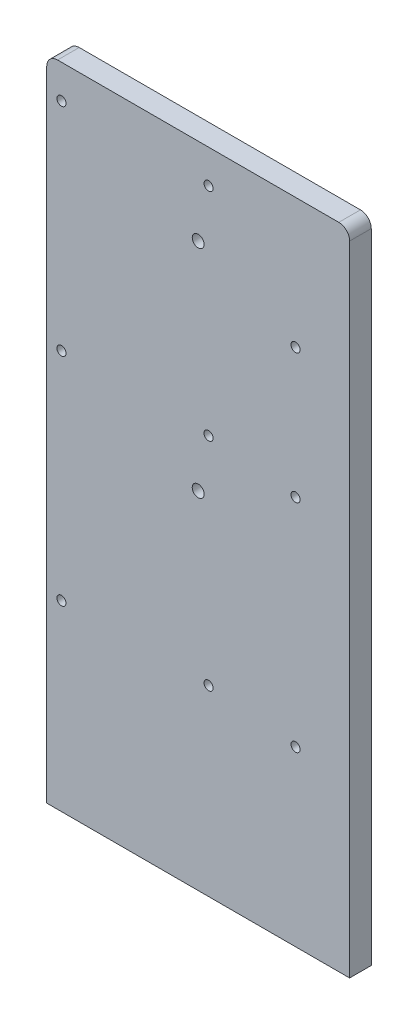
SolidWorks part; units mm, degrees
ref_plane "前视基准面" through (0, 0, 0) normal (0, 0, 1) x (1, 0, 0)
ref_plane "上视基准面" through (0, 0, 0) normal (0, 1, 0) x (1, 0, 0)
ref_plane "右视基准面" through (0, 0, 0) normal (1, 0, 0) x (0, 0, -1)
sketch "草图1" plane through (0, 0, 0) normal (0, 0, 1) x (1, 0, 0)
  line L1 (70, -150) -> (-70, -150)
  line L2 (70, -150) -> (70, 150)
  line L3 (70, 150) -> (-70, 150)
  line L4 (-70, -150) -> (-70, 150)
  line L5 (70, -150) -> (-70, 150) construction
  line L6 (70, 150) -> (-70, -150) construction
  point P0 (0, 0)
  dimension "D1" = 140
  dimension "D2" = 300
extrude "凸台-拉伸1" add sketch "草图1" along normal blind 10
hole_wizard "打孔尺寸(%根据)内六角圆柱头螺钉的类型1" positions "草图2" profile "草图3" counterbore size "M5" standard "GB"
sketch "草图2" plane through (0, 0, 0) normal (0, 0, -1) x (-1, 0, 0)
  point P0 (0, 110)
  point P3 (0, 10)
sketch "草图3" plane through (0, 110, 0) normal (1, 0, 0) x (0, 1, 0)
  line L0 (0, 0) -> (0, 16.0524)
  line L1 (0, 16.0524) -> (2.75, 14.4)
  line L2 (2.75, 14.4) -> (2.75, 5.7)
  line L3 (2.75, 5.7) -> (5, 5.7)
  line L4 (5, 5.7) -> (5, 0)
  line L5 (5, 0) -> (0, 0)
  line L10 (0, 16.0524) -> (-2.75, 14.4) construction
  line L11 (0, -6.35) -> (0, 107.95) construction
  dimension "孔直径" = 5.5
  dimension "孔深度" = 14.4
  dimension "柱形沉头孔直径" = 10
  dimension "柱形沉头孔深度" = 5.7
  dimension "导头角度" = 118
hole_wizard "M5 螺纹孔1" positions "草图4" profile "草图5" tap size "M5" standard "GB" end condition up to next
sketch "草图4" plane through (0, 0, 0) normal (0, 0, -1) x (-1, 0, 0)
  point P0 (-4.8, -65.5)
  point P3 (63.2, -65.5)
  point P6 (-4.8, 34.5)
  point P9 (63.2, 34.5)
  point P12 (-4.8, 134.5)
  point P15 (63.2, 134.5)
sketch "草图5" plane through (4.8, -65.5, 0) normal (1, 0, 0) x (0, 1, 0)
  line L0 (0, 0) -> (0, 10)
  line L1 (0, 10) -> (2.1, 10)
  line L2 (2.1, 10) -> (2.1, 0)
  line L5 (2.1, 0) -> (0, 0)
  line L11 (0, -6.35) -> (0, 107.95) construction
  dimension "通孔螺纹孔钻头直径" = 4.2
  dimension "通孔螺纹孔钻头深度" = 10
cosmetic thread "孔螺蚊线1"
cosmetic thread "孔螺蚊线2"
cosmetic thread "孔螺蚊线3"
cosmetic thread "孔螺蚊线4"
cosmetic thread "孔螺蚊线5"
cosmetic thread "孔螺蚊线6"
hole_wizard "M5 螺纹孔2" positions "草图6" profile "草图7" tap size "M5" standard "GB"
sketch "草图6" plane through (0, -150, 0) normal (0, -1, 0) x (-1, 0, 0)
  line L0 (-70, -5) -> (-50, -5) construction
  line L1 (-70, -10) -> (-70, 0) construction
  line L2 (-50, -5) -> (50, -5) construction
  line L5 (0, -5) -> (0, 0) construction
  point P0 (-50, -5)
  point P2 (50, -5)
  dimension "D1" = 100
cosmetic thread "孔螺蚊线7" parameters "D1"=10, "D2"=5
cosmetic thread "孔螺蚊线8" parameters "D1"=10, "D2"=5
sketch "草图7" plane through (50, -150, 5) normal (1, 0, 0) x (0, 0, -1)
  line L0 (0, 0) -> (0, 13.6618)
  line L1 (0, 13.6618) -> (2.1, 12.4)
  line L2 (2.1, 12.4) -> (2.1, 0)
  line L5 (2.1, 0) -> (0, 0)
  line L10 (0, 13.6618) -> (-2.1, 12.4) construction
  line L11 (0, -6.35) -> (0, 107.95) construction
  dimension "螺纹孔钻头直径" = 4.2
  dimension "螺纹孔钻头深度" = 12.4
  dimension "导头角度" = 118
hole_wizard "M5 螺纹孔3" positions "草图8" profile "草图9" tap size "M5" standard "GB" end condition up to next
sketch "草图8" plane through (0, 0, 10) normal (0, 0, 1) x (1, 0, 0)
  line L0 (45, -70) -> (45, 30) construction
  line L1 (45, 30) -> (45, 90) construction
  line L2 (45, 90) -> (45, 150) construction
  line L3 (70, 150) -> (-70, 150) construction
  line L6 (70, -150) -> (70, 150) construction
  point P0 (45, 90)
  point P2 (45, 30)
  point P4 (45, -70)
  dimension "D1" = 60
  dimension "D2" = 60
  dimension "D3" = 100
  dimension "D4" = 25
sketch "草图9" plane through (45, 90, 10) normal (1, 0, 0) x (0, -1, 0)
  line L0 (0, 0) -> (0, 10)
  line L1 (0, 10) -> (2.1, 10)
  line L2 (2.1, 10) -> (2.1, 0)
  line L5 (2.1, 0) -> (0, 0)
  line L11 (0, -6.35) -> (0, 107.95) construction
  dimension "通孔螺纹孔钻头直径" = 4.2
  dimension "通孔螺纹孔钻头深度" = 10
cosmetic thread "孔螺蚊线9"
cosmetic thread "孔螺蚊线10"
cosmetic thread "孔螺蚊线11"
fillet "圆角1" radius 5 2 edges at (-70, 150, 5) (70, 150, 5)
